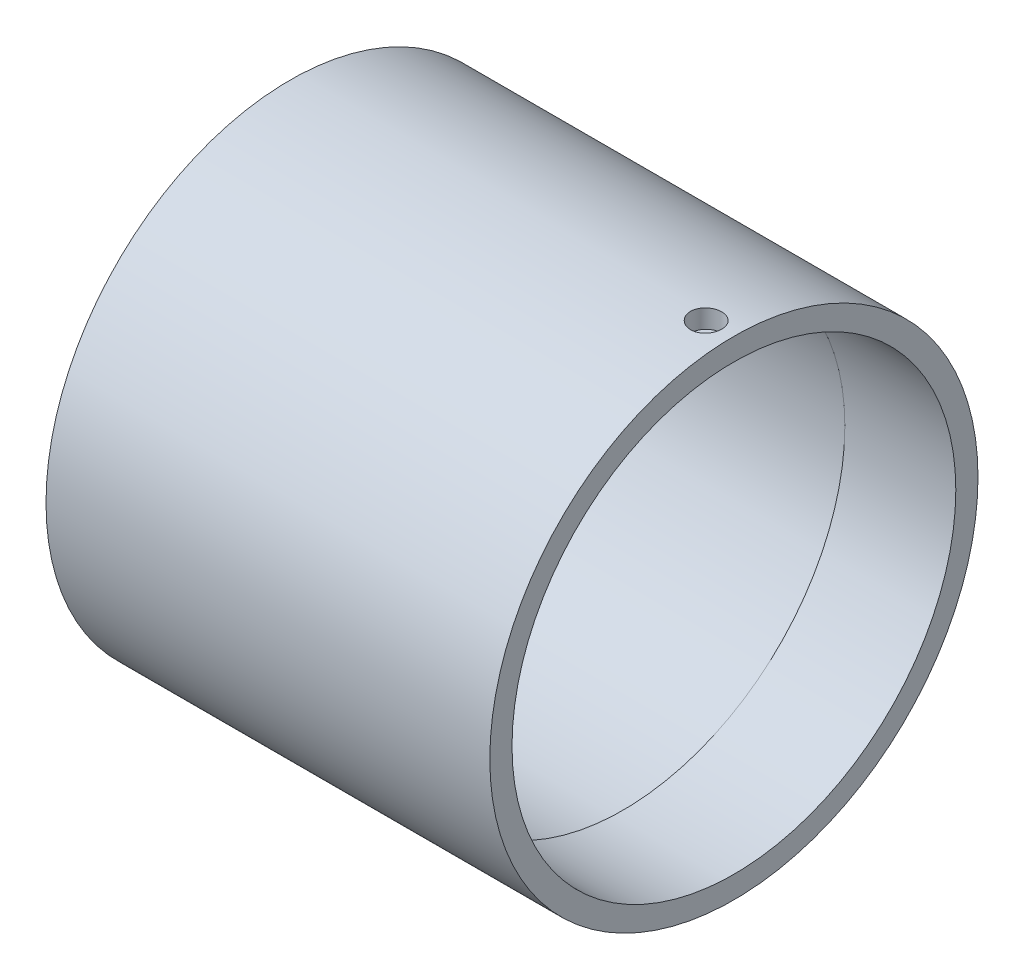
from build123d import *

# Parameters (mm, degrees)
SKETCH4_R          = 7
CUT_EXTRUDE1_DEPTH = 8.5
SKETCH5_R          = 4.25
CUT_EXTRUDE2_DEPTH = 8.5


with BuildPart() as part:
    # Sketch2 → Revolve1 (revolve)
    with BuildSketch(Plane.XY, mode=Mode.PRIVATE) as revolve1_sk:
        Polygon((-80.999754507, 110), (-80.999754507, 100), (-70.999754507, 100), (-70.999754507, 105), (-63.499754507, 105), (-63.499754507, 100), (-53.999754507, 100), (-53.999754507, 100.5), (69.000245493, 100.5), (69.000245493, 100), (119.000245493, 100), (119.000245493, 110), align=None)
    revolve(revolve1_sk.sketch.rotate(Axis((-113.629726069, 0, 0), (1, 0, 0)), 90), axis=Axis((-113.629726069, 0, 0), (1, 0, 0)))

    # Sketch4 → Cut-Extrude1 (cut)
    with BuildSketch(Plane(origin=(0, 110, 0), x_dir=(1, 0, 0), z_dir=(0, 1, 0))):
        with Locations(Location((106.500245493, 0, 0), (0, 0, 270))):
            Circle(SKETCH4_R)
    extrude(amount=-CUT_EXTRUDE1_DEPTH, mode=Mode.SUBTRACT)

    # Sketch5 → Cut-Extrude2 (cut)
    with BuildSketch(Plane(origin=(0, 101.5, 0), x_dir=(1, 0, 0), z_dir=(0, 1, 0))):
        with Locations(Location((106.500245493, 0, 0), (0, 0, 270))):
            Circle(SKETCH5_R)
    extrude(amount=-CUT_EXTRUDE2_DEPTH, mode=Mode.SUBTRACT)


solid = part.part
